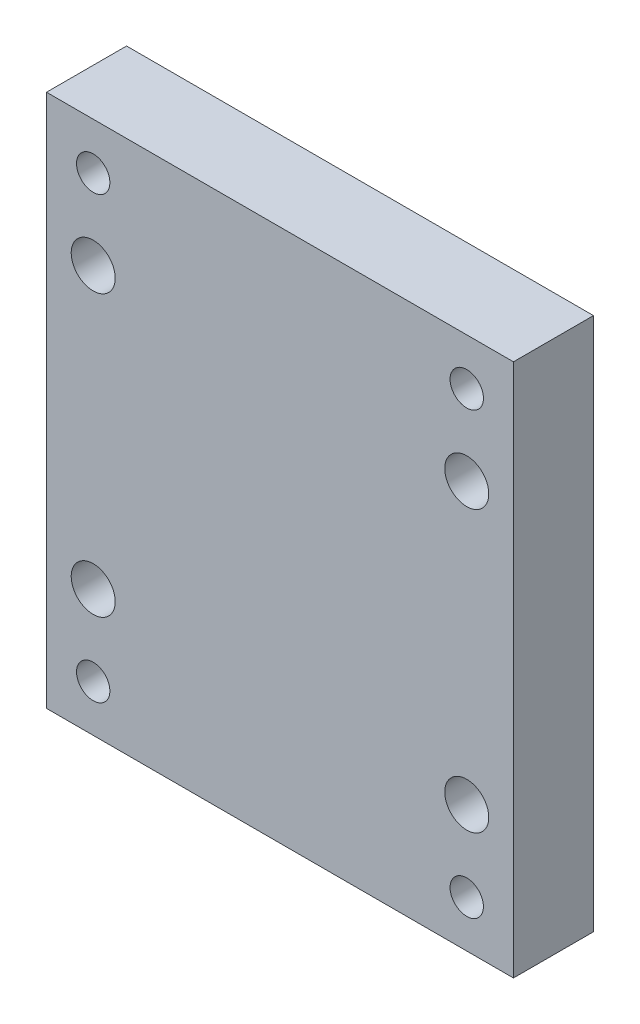
SolidWorks part; units mm, degrees
ref_plane "前视" through (0, 0, 0) normal (0, 0, 1) x (1, 0, 0)
ref_plane "上视" through (0, 0, 0) normal (0, 1, 0) x (1, 0, 0)
ref_plane "右视" through (0, 0, 0) normal (1, 0, 0) x (0, 0, -1)
sketch "草图1" plane through (0, 0, 0) normal (0, 0, 1) x (1, 0, 0)
  line L1 (-35, 40) -> (35, 40)
  line L2 (-35, 40) -> (-35, -40)
  line L3 (-35, -40) -> (35, -40)
  line L4 (35, 40) -> (35, -40)
  line L5 (-35, 40) -> (35, -40) construction
  line L6 (-35, -40) -> (35, 40) construction
  point P0 (0, 0)
  dimension "D1" = 70
  dimension "D2" = 80
extrude "凸台-拉伸1" add sketch "草图1" along normal blind 12
hole_wizard "M6 螺纹孔1" positions "草图3" profile "草图2" tap size "M6" standard "GB" end condition through all
sketch "草图3" plane through (0, 0, 0) normal (0, 0, -1) x (-1, 0, 0)
  point P0 (28, 33)
  point P3 (28, -33)
  point P6 (-28, -33)
  point P11 (-28, 33)
sketch "草图2" plane through (-28, 33, 0) normal (1, 0, 0) x (0, 1, 0)
  line L0 (0, 0) -> (0, 12)
  line L1 (0, 12) -> (2.5, 12)
  line L2 (2.5, 12) -> (2.5, 0)
  line L5 (2.5, 0) -> (0, 0)
  line L11 (0, -6.35) -> (0, 107.95) construction
  dimension "通孔螺纹孔钻头直径" = 5
  dimension "通孔螺纹孔钻头深度" = 12
cosmetic thread "孔螺蚊线1" parameters "D2"=6
cosmetic thread "孔螺蚊线2" parameters "D2"=6
cosmetic thread "孔螺蚊线3" parameters "D2"=6
cosmetic thread "孔螺蚊线4" parameters "D2"=6
hole_wizard "M6 六角凹头螺钉的柱形沉头孔1" positions "草图5" profile "草图4" counterbore size "M6" standard "ISO" end condition through all
sketch "草图5" plane through (0, 0, 0) normal (0, 0, -1) x (-1, 0, 0)
  line L0 (0, 0) -> (0, 40) construction
  line L1 (-35, 40) -> (35, 40) construction
  line L3 (-28, -21) -> (-28, 21) construction
  line L6 (-28, 0) -> (-35, 0) construction
  line L7 (-35, -40) -> (-35, 40) construction
  point P0 (-28, -21)
  point P2 (-28, 21)
  point P21 (28, -21)
  point P22 (28, 21)
  dimension "D1" = 7
  dimension "D2" = 42
sketch "草图4" plane through (28, -21, 0) normal (1, 0, 0) x (0, 1, 0)
  line L0 (0, 0) -> (0, 12)
  line L1 (0, 12) -> (3.3, 12)
  line L3 (3.3, 12) -> (3.3, 6.4)
  line L4 (3.3, 6.4) -> (5.5, 6.4)
  line L5 (5.5, 6.4) -> (5.5, 0)
  line L7 (5.5, 0) -> (0, 0)
  line L11 (0, -6.35) -> (0, 107.95) construction
  dimension "通孔孔直径" = 6.6
  dimension "通孔孔深度" = 12
  dimension "柱形沉头孔直径" = 11
  dimension "柱形沉头孔深度" = 6.4
